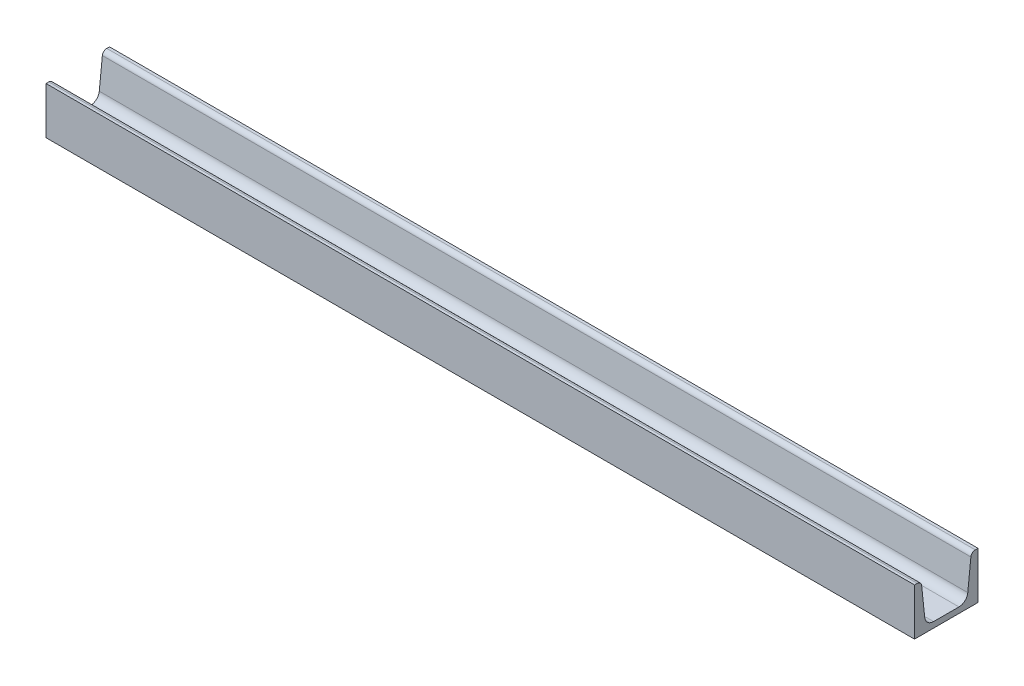
SolidWorks part; units mm, degrees
material "AISI 304"
ref_plane "Front Plane" through (0, 0, 0) normal (0, 0, 1) x (1, 0, 0)
ref_plane "Top Plane" through (0, 0, 0) normal (0, 1, 0) x (1, 0, 0)
ref_plane "Right Plane" through (0, 0, 0) normal (1, 0, 0) x (0, 0, -1)
other "Configuration Table"
sketch "草图1" plane through (0, 0, 0) normal (0, 0, 1) x (1, 0, 0)
  line L0 (-342, 0) -> (342, 0)
  point P4 (0, 0)
  dimension "D1" = 684
other "GB/T 707-1988 hot-rolled channel 05(1)"
ref_plane "Plane1" through (-342, 0, 0) normal (1, 0, 0) x (0, 1, 0)
sketch "Sketch1" plane through (-342, 0, 0) normal (1, 0, 0) x (0, 1, 0)
  line L0 (37, 50) -> (0, 50)
  line L1 (37, 0) -> (0, 0)
  line L2 (0, 50) -> (0, 0)
  line L3 (-9.5694, 25) -> (49.7414, 25) construction
  line L4 (4.5, 34.9892) -> (4.5, 15.0108)
  line L5 (37, 0) -> (37, 2.1406)
  line L6 (37, 50) -> (37, 47.8594)
  line L7 (10.7683, 8.0491) -> (33.8658, 5.6215)
  line L17 (10.7683, 41.9509) -> (33.8658, 44.3785)
  arc A0 (33.8658, 44.3785) -> (37, 47.8594) centre (33.5, 47.8594) ccw
  arc A1 (33.8658, 5.6215) -> (37, 2.1406) centre (33.5, 2.1406) cw
  arc A2 (4.5, 15.0108) -> (10.7683, 8.0491) centre (11.5, 15.0108) ccw
  arc A10 (4.5, 34.9892) -> (10.7683, 41.9509) centre (11.5, 34.9892) cw
  point P6 (0, 0)
  point P8 (0, 25)
  point P9 (4.5, 25.8841)
  point P10 (18.5, 50)
  point P13 (37, 44.7079)
  point P14 (20.75, 43)
  point P19 (4.5, 25)
equation "\"RI@Sketch1\" = \"D1@Sketch1\""
equation "\"D3@Sketch1\" =  ( \"BF@Sketch1\" - \"D6@Sketch1\" )  / 2"
